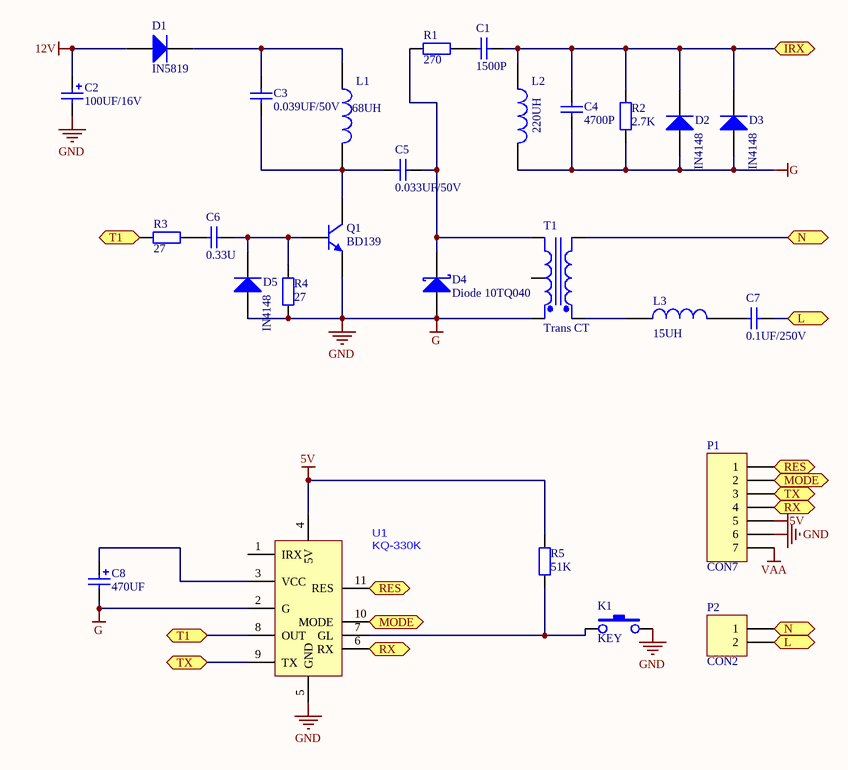
[diagram p0: MISC76200-3.SchDoc]
# Altium project MISC76200-2.PrjPcb
1 sheet, 27 parts. Net scope: flat (ports and power ports of the same name join across sheets).
Board file: MISC76200.PcbDoc

## Sheet MISC76200-3.SchDoc
size A4

### Parts
C1  1500P  [RAD-0.3]
C2  100UF/16V  [POLAR0.8]
C3  0.039UF/50V  [RAD-0.3]
C4  4700P  [RAD-0.3]
C5  0.033UF/50V  [RAD-0.3]
C6  0.33U  [RAD-0.3]
C7  0.1UF/250V  [RAD-0.3]
C8  470UF  [POLAR0.8]
D1  IN5819  [DO-35A]
D2  IN4148  [DO-35A]
D3  IN4148  [DO-35A]
D4  Diode 10TQ040  [TO-220AC]
D5  IN4148  [DO-35A]
K1  KEY  [DIP-3X6X4.3]
L1  68UH  [AL0204]
L2  220UH  [AL0204]
L3  15UH  [AL0204]
P1  CON7  [HDR1X7]
P2  CON2  [HDR1X2]
Q1  BD139  [TO-226-AA]
R1  270  [AXIAL-0.4]
R2  2.7K  [AXIAL-0.4]
R3  27  [AXIAL-0.4]
R4  27  [AXIAL-0.4]
R5  51K  [AXIAL-0.4]
T1  Trans CT  [TRF_5]
U1  KQ-330K  [20130-10PIN]

### Ports
IRX (bidir), L, MODE (bidir), N (bidir), RES (bidir), RX (bidir), T1 (bidir), TX (bidir)

### Nets
5V: P1.5 R5.2 U1.4(5V)
12V: C2.1 D1.1(A)
G: C2.2 C4.2 C8.2 D2.1(A) D3.1(A) D4.3(A) D5.1(A) K1.3 L2.2 P1.6 Q1.3(E) R2.1 R4.1 T1.3(Sec+) U1.2(G) U1.5(GND)  [also labelled GND]
VAA: P1.7
NetC1_1: C1.1 C4.1 D2.2(K) D3.2(K) L2.1 R2.2 ; port IRX
NetC1_2: C1.2 R1.2
NetC3_1: C3.1 C5.2 L1.2 Q1.1(C)
NetC3_2: C3.2 D1.2(K) L1.1
NetC5_1: C5.1 D4.1(K) R1.1 T1.5(Sec-)
NetC6_1: C6.1 D5.2(K) Q1.2(B) R4.2
NetC6_2: C6.2 R3.2
NetC7_1: C7.1 P2.2 ; port L
NetC7_2: C7.2 L3.2
NetC8_1: C8.1 U1.3(VCC)
NetK1_1: K1.1 R5.1 U1.7(GL)
NetL3_1: L3.1 T1.1(Pri+)
NetP1_1: P1.1 U1.11(RES) ; port RES
NetP1_2: P1.2 U1.10(MODE) ; port MODE
NetP1_3: P1.3 U1.9(TX) ; port TX
NetP1_4: P1.4 U1.6(RX) ; port RX
NetP2_1: P2.1 T1.2(Pri-) ; port N
NetR3_1: R3.1 U1.8(OUT) ; port T1

Not connected (* = marked no-connect by the designer): T1 4(SecCT); U1 1(IRX)

### Library data of the parts
C1 C3-C7 = Cap: Capacitor; Value: 100pF; Published: 8-Jun-2000; LatestRevisionDate: 17-Jul-2002; LatestRevisionNote: Re-released for DXP Platform.; PackageReference: RAD-0.3; PackageDescription: Radial Cap, Thru-Hole; 2 Leads; 0.3 in Pin Spacing; Publisher: Altium Limited
C2 C8 = Cap Pol2: Polarized Capacitor (Axial); Value: 100pF; Published: 8-Jun-2000; LatestRevisionDate: 17-Jul-2002; LatestRevisionNote: Re-released for DXP Platform.; PackageReference: POLAR0.8; PackageDescription: Polarized Capacitor; 2 Leads; Publisher: Altium Limited
D1-D3 D5 = Diode 1N4149: Computer Diode; Published: 8-Jun-2000; LatestRevisionDate: 17-Jul-2002; LatestRevisionNote: Re-released for DXP Platform.; DatasheetVersion: 1989; PackageVersion: 1989; PackageReference: DO-35A; PackageDescription: Diode, Axial; Body 4.6 x 1.9 mm (LxDia. max), Lead Dia. 0.53 mm (max); Code_JEDEC: DO-204-AH; ComponentLink1Description: Manufacturer Link; ComponentLink1URL: http://www.national.com/; Publisher: Altium Limited
D4 = Diode 10TQ040: Schottky Rectifier; Note: Terminal 2 is the TAB and is electrically connected to the cathode; Published: 8-Jun-2000; LatestRevisionDate: 17-Jul-2002; LatestRevisionNote: Re-released for DXP Platform.; DatasheetVersion: PD-2.057B; PackageVersion: Feb-1998; PackageReference: TO-220AC; PackageDescription: TO, Thru-Hole, Vertical, Heatsink Mounted; 3 In-Line Leads (1 Absent); Pitch 2.54 mm; ComponentLink1Description: Manufacturer Link; ComponentLink1URL: http://www.irf.com/; Publisher: Altium Limited
L1-L3 = INDUCTOR
P1 = Header 7: Header, 7-Pin; LatestRevisionDate: 17-Jul-2002; LatestRevisionNote: Re-released for DXP Platform.; Publisher: Altium Limited
P2 = Header 2: Header, 2-Pin; LatestRevisionDate: 17-Jul-2002; LatestRevisionNote: Re-released for DXP Platform.; Publisher: Altium Limited
Q1 = NPN: NPN Bipolar Transistor; Published: 8-Jun-2000; LatestRevisionDate: 17-Jul-2002; LatestRevisionNote: Re-released for DXP Platform.; PackageReference: TO-226-AA; PackageDescription: TO, Flat Index; 3 In-Line, Axial Leads; Body Dia. 4.8mm; Leads 0.55 x 0.51 mm (max); Code_JEDEC: TO-226-AA; Publisher: Altium Limited
R1-R5 = Res2: Resistor; Value: 1K; Published: 8-Jun-2000; LatestRevisionDate: 17-Jul-2002; LatestRevisionNote: Re-released for DXP Platform.; PackageReference: AXIAL-0.4; PackageDescription: Axial Device, Thru-Hole; 2 Leads; 0.4 in Pin Spacing; Publisher: Altium Limited
T1 = Trans CT: Center-Tapped Transformer (Coupled Inductor Model); Published: 8-Jun-2000; LatestRevisionDate: 17-Jul-2002; LatestRevisionNote: Re-released for DXP Platform.; PackageReference: TRF_5; PackageDescription: Transformer; 5 Leads; Publisher: Altium Limited
U1 = 20130-10PIN